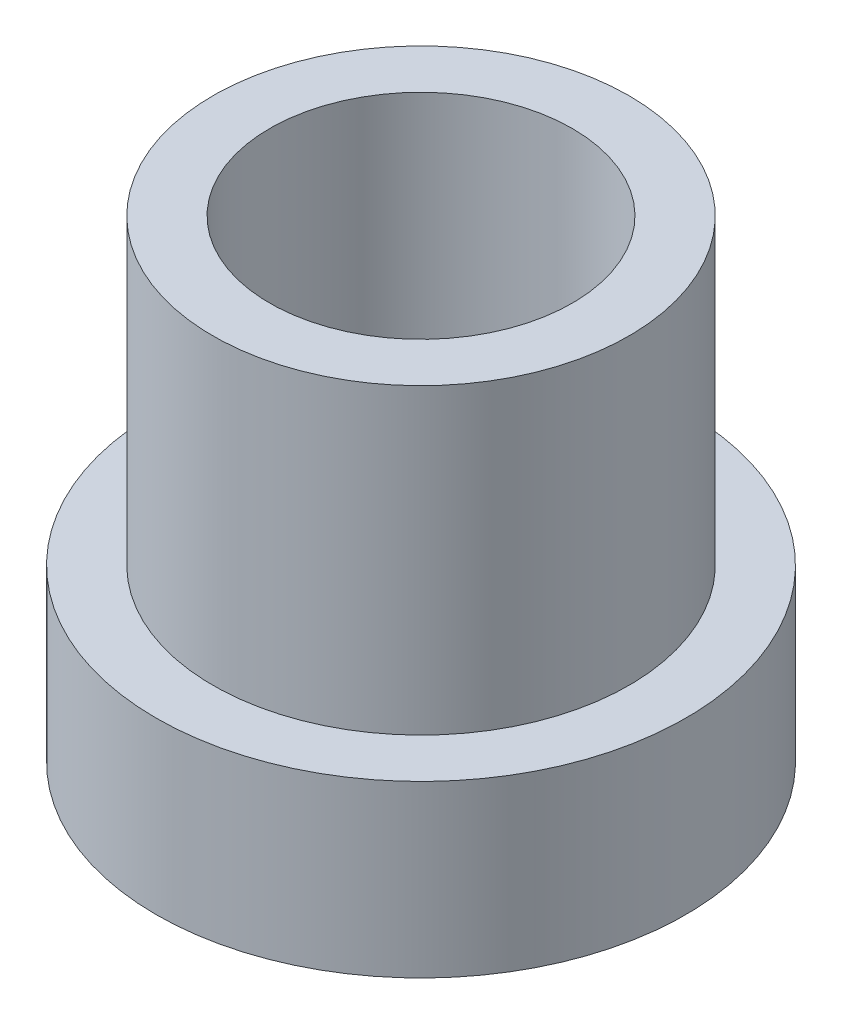
SolidWorks part; units mm, degrees
ref_plane "前视基准面" through (0, 0, 0) normal (0, 0, 1) x (1, 0, 0)
ref_plane "上视基准面" through (0, 0, 0) normal (0, 1, 0) x (1, 0, 0)
ref_plane "右视基准面" through (0, 0, 0) normal (1, 0, 0) x (0, 0, -1)
sketch "草图1" plane through (0, 0, 0) normal (0, 0, 1) x (1, 0, 0)
  line L0 (0, 0) -> (0, 5883.4077) construction
  line L1 (4, 7.2614) -> (5.5, 7.2614)
  line L2 (5.5, 7.2614) -> (5.5, -0.7386)
  line L3 (5.5, -0.7386) -> (7, -0.7386)
  line L4 (7, -0.7386) -> (7, -5.2386)
  line L5 (7, -5.2386) -> (4, -5.2386)
  line L6 (4, -5.2386) -> (4, 7.2614)
  dimension "D1" = 4
  dimension "D2" = 12.5
  dimension "D3" = 1.5
  dimension "D4" = 8
  dimension "D5" = 1.5
revolve "旋转1" add sketch "草图1" angle 360 about L0
sketch "草图2" plane through (0, 0, 0) normal (0, 0, 1) x (1, 0, 0)
  line L0 (-7, -5.2386) -> (7, -5.2386) construction
  circle A0 centre (0, -2.9886) radius 1.5
  dimension "D1" = 3
  dimension "D2" = 2.25
extrude "切除-拉伸1" cut sketch "草图2" against normal blind 10
